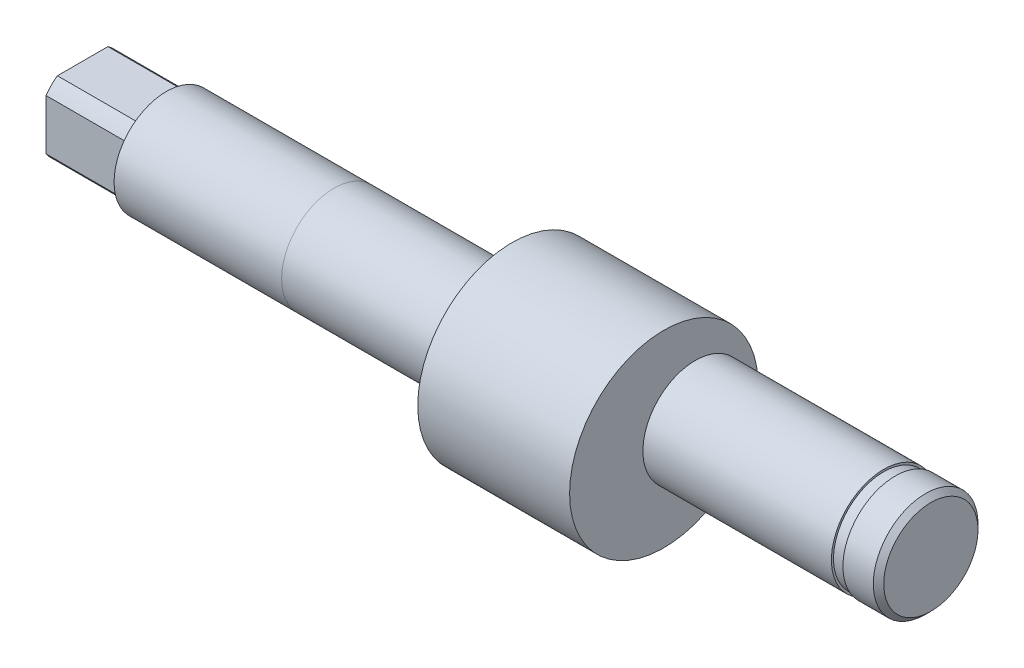
from build123d import *

# Parameters (mm, degrees)
SKETCH_2_R      = 9
EXTRUDE_1_DEPTH = 14.5
SKETCH_3_R      = 5
EXTRUDE_2_DEPTH = 18
SKETCH_4_R      = 4.8
EXTRUDE_3_DEPTH = 1.1
SKETCH_5_R      = 5
EXTRUDE_4_DEPTH = 3.4
CHAMFER_1_SIZE  = 0.5
SKETCH_6_R      = 5
EXTRUDE_5_DEPTH = 17
SKETCH_7_R      = 5
EXTRUDE_6_DEPTH = 16
EXTRUDE_7_DEPTH = 8


with BuildPart() as part:
    # 草图2 → 凸台-拉伸1 (new body)
    with BuildSketch(Plane(origin=(0, 0, 0), x_dir=(0, 0, -1), z_dir=(1, 0, 0))):
        with Locations(Location((0, 0, 0), (0, 0, 180))):
            Circle(SKETCH_2_R)
    extrude(amount=EXTRUDE_1_DEPTH)

    # 草图3 → 凸台-拉伸2 (add)
    with BuildSketch(Plane(origin=(14.5, 0, 0), x_dir=(0, 0, -1), z_dir=(1, 0, 0))):
        with Locations((3, 0)):
            Circle(SKETCH_3_R)
    extrude(amount=EXTRUDE_2_DEPTH)

    # 草图4 → 凸台-拉伸3 (add)
    with BuildSketch(Plane(origin=(32.5, 0, 0), x_dir=(0, 0, -1), z_dir=(1, 0, 0))):
        with Locations((3, 0)):
            Circle(SKETCH_4_R)
    extrude(amount=EXTRUDE_3_DEPTH)

    # 草图5 → 凸台-拉伸4 (add)
    with BuildSketch(Plane(origin=(33.6, 0, 0), x_dir=(0, 0, -1), z_dir=(1, 0, 0))):
        with Locations((3, 0)):
            Circle(SKETCH_5_R)
    extrude(amount=EXTRUDE_4_DEPTH)

    # 倒角1
    chamfer_1_edges = [part.edges().sort_by_distance(p)[0] for p in [
        (37, 0, 2),
    ]]
    chamfer(chamfer_1_edges, length=CHAMFER_1_SIZE)

    # 草图6 → 凸台-拉伸5 (add)
    with BuildSketch(Plane.ZY):
        Circle(SKETCH_6_R)
    extrude(amount=EXTRUDE_5_DEPTH)


with BuildPart() as body_2:
    # 草图7 → 凸台-拉伸6 (new body)
    with BuildSketch(Plane.ZY.offset(17)):
        Circle(SKETCH_7_R)
    extrude(amount=EXTRUDE_6_DEPTH)

    # 草图8 → 凸台-拉伸7 (add)
    with BuildSketch(Plane.ZY.offset(33)):
        with BuildLine():
            Line((-2.41091269, -3.5), (2.41091269, -3.5))
            ThreePointArc((2.41091269, -3.5), (3.00520382, -3.00520382), (3.5, -2.41091269))
            Line((3.5, -2.41091269), (3.5, 2.41091269))
            ThreePointArc((3.5, 2.41091269), (3.00520382, 3.00520382), (2.41091269, 3.5))
            Line((2.41091269, 3.5), (-2.41091269, 3.5))
            ThreePointArc((-2.41091269, 3.5), (-3.00520382, 3.00520382), (-3.5, 2.41091269))
            Line((-3.5, 2.41091269), (-3.5, -2.41091269))
            ThreePointArc((-3.5, -2.41091269), (-3.00520382, -3.00520382), (-2.41091269, -3.5))
        make_face()
    extrude(amount=EXTRUDE_7_DEPTH)


solid = Compound([part.part, body_2.part])
